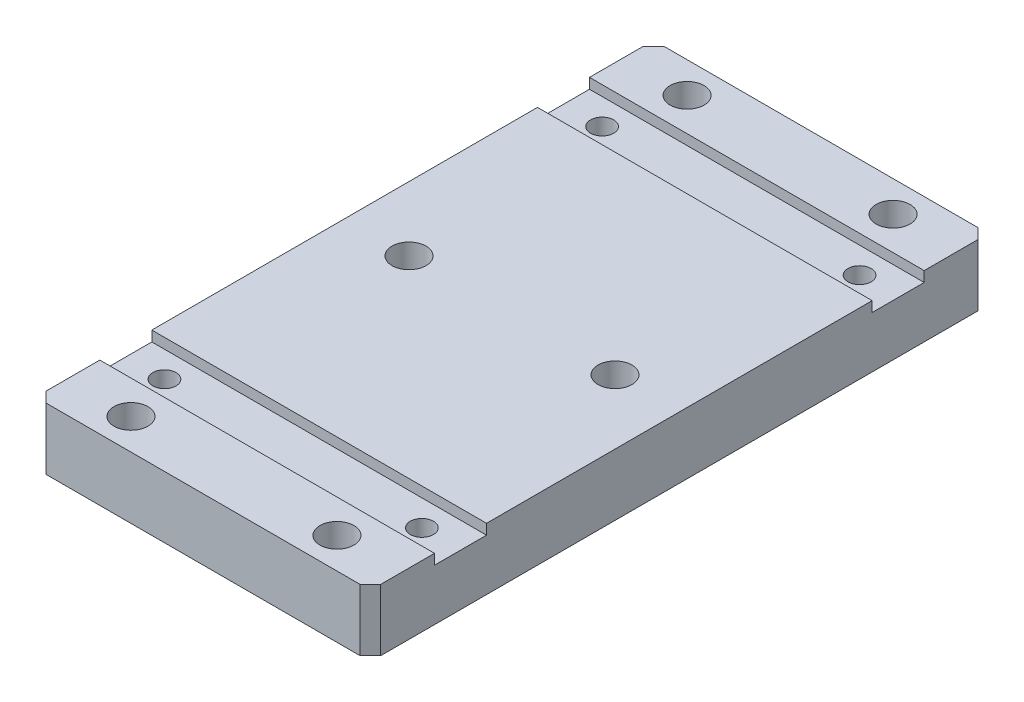
SolidWorks part; units mm, degrees
material "A6061"
ref_plane "前基準面" through (0, 0, 0) normal (0, 0, 1) x (1, 0, 0)
ref_plane "上基準面" through (0, 0, 0) normal (0, 1, 0) x (1, 0, 0)
ref_plane "右基準面" through (0, 0, 0) normal (1, 0, 0) x (0, 0, -1)
sketch "草图1" plane through (0, 0, 0) normal (0, 1, 0) x (1, 0, 0)
  line L1 (-32.5, 60) -> (32.5, 60)
  line L2 (-32.5, 60) -> (-32.5, -60)
  line L3 (-32.5, -60) -> (32.5, -60)
  line L4 (32.5, 60) -> (32.5, -60)
  line L5 (-32.5, 60) -> (32.5, -60) construction
  line L6 (-32.5, -60) -> (32.5, 60) construction
  point P0 (0, 0)
  dimension "D1" = 120
  dimension "D2" = 65
extrude "凸台-拉伸1" add sketch "草图1" along normal blind 12
hole_wizard "M6 间隙孔1" positions "草图2" profile "草图3" hole size "M6" standard "GB" end condition up to next
sketch "草图2" plane through (0, 12, 0) normal (0, 1, 0) x (1, 0, 0)
  line L0 (0, 0) -> (0, -66.7428) construction
  line L2 (0, 0) -> (-33.1819, 0) construction
  point P0 (-20, -54)
  point P12 (20, -54)
  point P18 (-20, 0)
  point P19 (20, 0)
  point P20 (-20, 54)
  point P21 (20, 54)
  dimension "D1" = 3
  dimension "D2" = 40
  dimension "D3" = 54
sketch "草图3" plane through (-20, 12, 54) normal (1, 0, 0) x (0, 0, 1)
  line L0 (0, 0) -> (0, 12)
  line L1 (0, 12) -> (3.3, 12)
  line L2 (3.3, 12) -> (3.3, 0)
  line L5 (3.3, 0) -> (0, 0)
  line L11 (0, -6.35) -> (0, 107.95) construction
  dimension "通孔孔直径" = 6.6
  dimension "通孔孔深度" = 12
sketch "草图4" plane through (0, 12, 0) normal (0, 1, 0) x (1, 0, 0)
  line L5 (0, 0) -> (-33.9185, 0) construction
  line L8 (32.5, 47.55) -> (-32.5, 47.55)
  line L9 (32.5, 47.55) -> (32.5, 37.45)
  line L10 (32.5, 37.45) -> (-32.5, 37.45)
  line L11 (-32.5, 47.55) -> (-32.5, 37.45)
  line L13 (32.5, -60) -> (32.5, 60) construction
  line L14 (-32.5, 60) -> (-32.5, -60) construction
  line L15 (-32.5, -47.55) -> (-32.5, -37.45)
  line L16 (32.5, -37.45) -> (-32.5, -37.45)
  line L17 (32.5, -47.55) -> (32.5, -37.45)
  line L18 (32.5, -47.55) -> (-32.5, -47.55)
  dimension "D1" = 85
  dimension "D2" = 10.1
extrude "切除-拉伸1" cut sketch "草图4" against normal blind 2
chamfer "倒角1" distance 2 angle 45 4 edges at (-32.5, 6, -60) (32.5, 6, -60) (32.5, 6, 60) (-32.5, 6, 60)
sketch "草图9" plane through (0, 0, 0) normal (0, -1, 0) x (-1, 0, 0)
  line L0 (0, 87.3946) -> (0, 0) construction
  line L1 (0, 0) -> (-45.1412, 0) construction
  line L4 (-32.5, 42.5) -> (-23.5585, 42.5) construction
  line L5 (-32.5, -58) -> (-32.5, 58) construction
  line L7 (-32.5, 37.45) -> (-32.5, 47.55) construction
  point P0 (-25, 42.5)
  point P10 (-25, -42.5)
  point P11 (25, -42.5)
  point P12 (25, 42.5)
  dimension "D1" = 50
hole_wizard "M4 六角圆柱头螺钉的柱形沉头孔1" positions "草图9" profile "草图10" counterbore size "M4" standard "GB" end condition up to next
sketch "草图10" plane through (25, 0, -42.5) normal (1, 0, 0) x (0, 0, -1)
  line L0 (0, 0) -> (0, 10)
  line L1 (0, 10) -> (2.25, 10)
  line L3 (2.25, 10) -> (2.25, 4.6)
  line L4 (2.25, 4.6) -> (4, 4.6)
  line L5 (4, 4.6) -> (4, 0)
  line L7 (4, 0) -> (0, 0)
  line L11 (0, -6.35) -> (0, 107.95) construction
  dimension "通孔孔直径" = 4.5
  dimension "通孔孔深度" = 10
  dimension "柱形沉头孔直径" = 8
  dimension "柱形沉头孔深度" = 4.6
